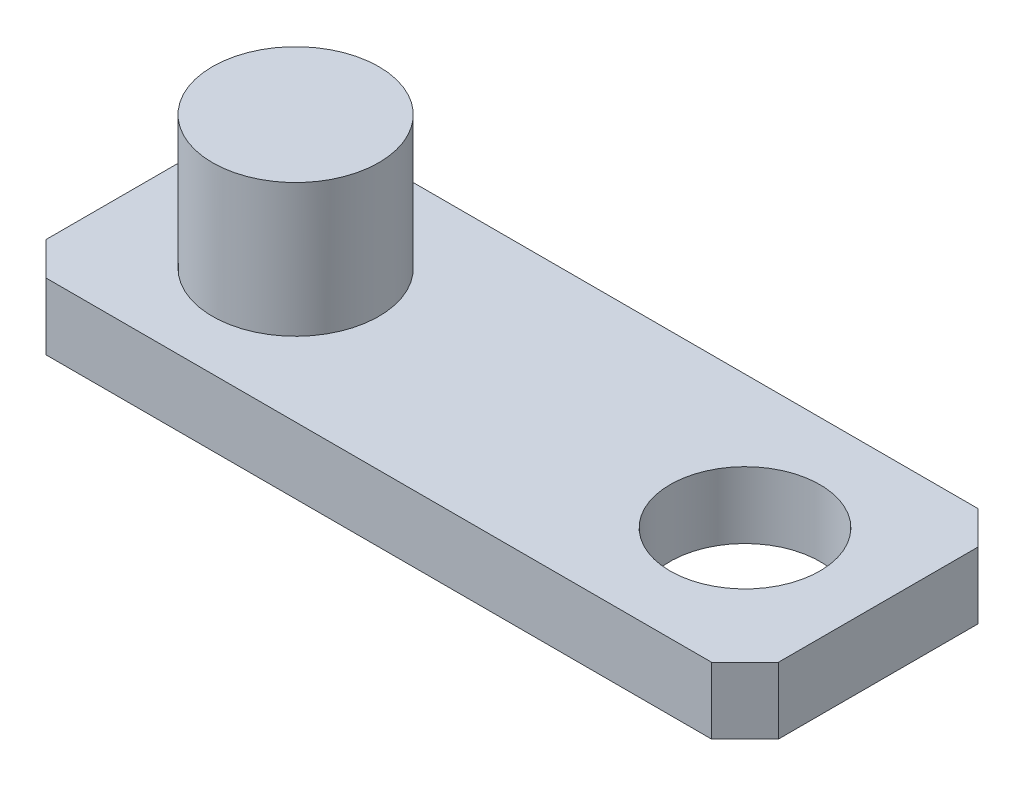
from build123d import *

# Parameters (mm, degrees)
SKETCH1_W           = 22
SKETCH1_H           = 8
BOSS_EXTRUDE1_DEPTH = 2
SKETCH2_R           = 2.25
CUT_EXTRUDE1_DEPTH  = 12.874342087
SKETCH3_R           = 2.5
BOSS_EXTRUDE2_DEPTH = 4
CHAMFER1_SIZE       = 1


with BuildPart() as part:
    # Sketch1 → Boss-Extrude1 (new body)
    with BuildSketch(Plane(origin=(0, 0, 0), x_dir=(1, 0, 0), z_dir=(0, 1, 0))):
        Rectangle(SKETCH1_W, SKETCH1_H)
    extrude(amount=BOSS_EXTRUDE1_DEPTH)

    # Sketch2 → Cut-Extrude1 (cut, through all)
    with BuildSketch(Plane(origin=(0, 2, 0), x_dir=(1, 0, 0), z_dir=(0, 1, 0))):
        with Locations(Location((7, 0, 0), (0, 0, 270))):
            Circle(SKETCH2_R)
    extrude(amount=-CUT_EXTRUDE1_DEPTH, mode=Mode.SUBTRACT)

    # Sketch3 → Boss-Extrude2 (add)
    with BuildSketch(Plane(origin=(0, 2, 0), x_dir=(1, 0, 0), z_dir=(0, 1, 0))):
        with Locations(Location((-6.5, 0, 0), (0, 0, 90))):
            Circle(SKETCH3_R)
    extrude(amount=BOSS_EXTRUDE2_DEPTH)

    # Chamfer1
    chamfer1_edges = [part.edges().sort_by_distance(p)[0] for p in [
        (11, 1, 4),
        (-11, 1, 4),
        (-11, 1, -4),
        (11, 1, -4),
    ]]
    chamfer(chamfer1_edges, length=CHAMFER1_SIZE)


solid = part.part
